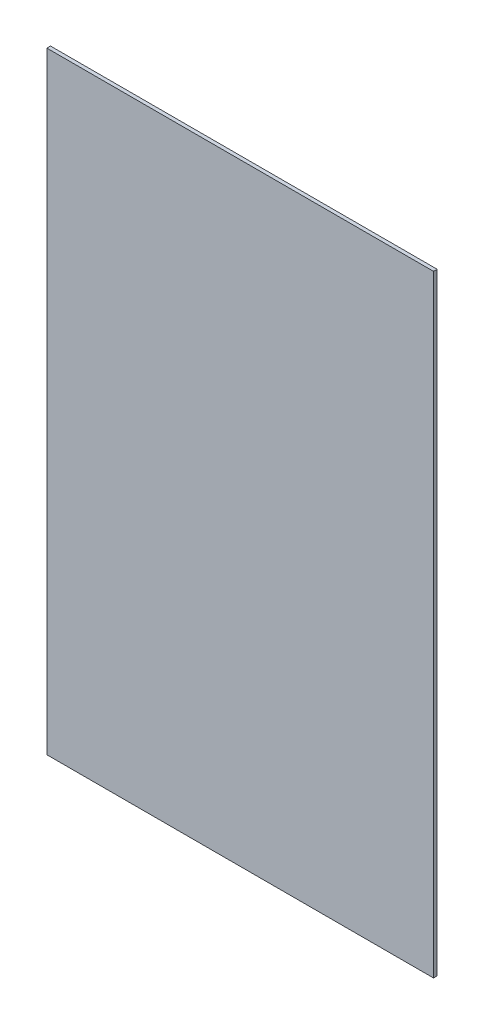
SolidWorks part; units mm, degrees
material "PMMA(有机玻璃)"
ref_plane "前视" through (0, 0, 0) normal (0, 0, 1) x (1, 0, 0)
ref_plane "上视" through (0, 0, 0) normal (0, 1, 0) x (1, 0, 0)
ref_plane "右视" through (0, 0, 0) normal (1, 0, 0) x (0, 0, -1)
sketch "草图1" plane through (0, 0, 0) normal (0, 0, 1) x (1, 0, 0)
  line L1 (-266, 421) -> (266, 421)
  line L2 (-266, 421) -> (-266, -421)
  line L3 (-266, -421) -> (266, -421)
  line L4 (266, 421) -> (266, -421)
  line L5 (-266, 421) -> (266, -421) construction
  line L6 (-266, -421) -> (266, 421) construction
  point P0 (0, 0)
  dimension "D1" = 842
  dimension "D2" = 532
extrude "凸台-拉伸1" add sketch "草图1" along normal blind 5
hole_wizard "M5 间隙孔1" positions "草图3" profile "草图2" hole size "M5" standard "GB"
sketch "草图3" plane through (0, 0, 5) normal (0, 0, 1) x (1, 0, 0)
  line L0 (-427.5, 273) -> (-427.5, -273) construction
  line L1 (-427.5, -273) -> (427.5, -273) construction
  line L2 (0, 273) -> (0, -273) construction
  line L3 (427.5, 273) -> (-427.5, 273) construction
  line L5 (-427.5, 0) -> (427.5, 0) construction
  line L6 (427.5, -273) -> (427.5, 273) construction
  point P0 (-375, -261)
  point P46 (415.5, 250)
  point P48 (-415.5, 250)
  point P58 (-125, -261)
  point P59 (125, -261)
  point P61 (-125, 261)
  point P62 (125, 261)
  point P64 (-375, 261)
  point P88 (375, -261)
  point P89 (375, 261)
  point P108 (415.5, 0)
  point P109 (-415.5, 0)
  point P110 (415.5, -250)
  point P111 (-415.5, -250)
  dimension "D1" = 12
  dimension "D2" = 12
  dimension "D5" = 3
  dimension "D3" = 12
  dimension "D6" = 4
  dimension "D4" = 2
sketch "草图2" plane through (-375, -261, 5) normal (1, 0, 0) x (0, -1, 0)
  line L0 (0, 0) -> (0, 5)
  line L1 (0, 5) -> (2.75, 5)
  line L2 (2.75, 5) -> (2.75, 0)
  line L5 (2.75, 0) -> (0, 0)
  line L11 (0, -6.35) -> (0, 107.95) construction
  dimension "通孔孔直径" = 5.5
  dimension "通孔孔深度" = 5
